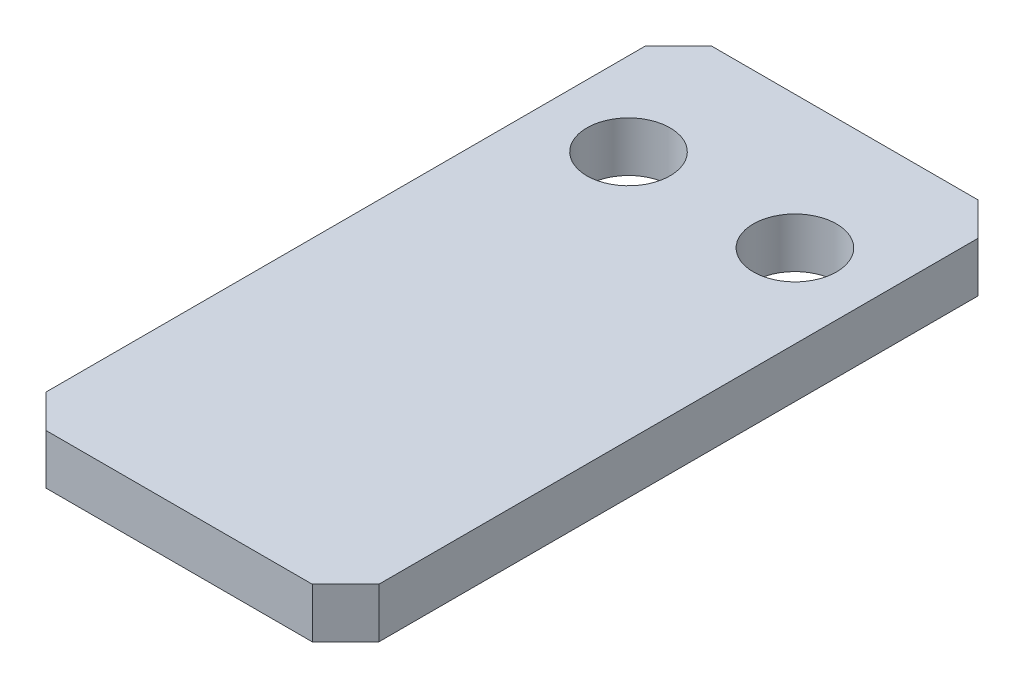
SolidWorks part; units mm, degrees
ref_plane "Front Plane" through (0, 0, 0) normal (0, 0, 1) x (1, 0, 0)
ref_plane "Top Plane" through (0, 0, 0) normal (0, 1, 0) x (1, 0, 0)
ref_plane "Right Plane" through (0, 0, 0) normal (1, 0, 0) x (0, 0, -1)
sketch "Sketch1" plane through (0, 0, 0) normal (0, 1, 0) x (1, 0, 0)
  line L1 (-5, 10) -> (5, 10)
  line L2 (-5, 10) -> (-5, -10)
  line L3 (-5, -10) -> (5, -10)
  line L4 (5, 10) -> (5, -10)
  line L5 (-5, 10) -> (5, -10) construction
  line L6 (-5, -10) -> (5, 10) construction
  point P0 (0, 0)
  dimension "D1" = 10
  dimension "D2" = 20
extrude "Boss-Extrude1" add sketch "Sketch1" along normal blind 1.5
chamfer "Chamfer1" distance 1 angle 45 4 edges at (5, 0.75, 10) (5, 0.75, -10) (-5, 0.75, -10) (-5, 0.75, 10)
hole_wizard "Ø2.5 (2.5) Diameter Hole1" positions "3DSketch1" profile "Sketch2" hole size "Ø2.5" standard "Gb"
sketch3d "3DSketch1"
  point P0 (-2.5, 1.5, -6)
  point P3 (2.5, 1.5, -6)
  dimension "D1" = 2.5
  dimension "D2" = 2.5
  dimension "D3" = 4
sketch "Sketch2" plane through (-2.5, 1.5, -6) normal (1, 0, 0) x (0, 0, 1)
  line L0 (0, 0) -> (0, 10.7511)
  line L1 (0, 10.7511) -> (1.25, 10)
  line L2 (1.25, 10) -> (1.25, 0)
  line L5 (1.25, 0) -> (0, 0)
  line L10 (0, 10.7511) -> (-1.25, 10) construction
  line L11 (0, -6.35) -> (0, 107.95) construction
  dimension "孔直径" = 2.5
  dimension "孔深度" = 10
  dimension "导头角度" = 118
